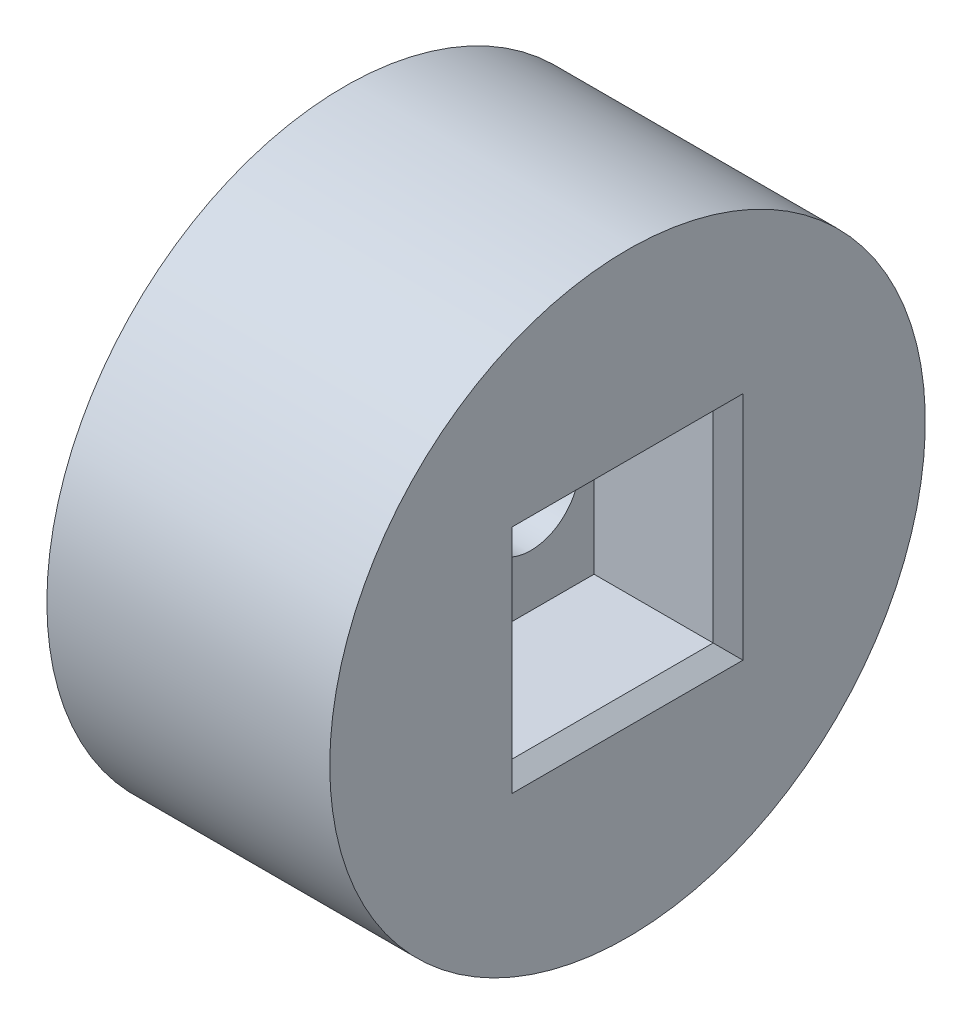
from build123d import *

# Parameters (mm, degrees)
SKETCH1_W                                           = 19
SKETCH1_H                                           = 20
SKETCH2_W                                           = 13.5
SKETCH2_H                                           = 13.5
CUT_EXTRUDE1_DEPTH                                  = 9
CBORE_FOR_M3_HEX_SOCKET_HEAD_CAP_SCREW1_D           = 3.4
CBORE_FOR_M3_HEX_SOCKET_HEAD_CAP_SCREW1_CBORE_D     = 6.5
CBORE_FOR_M3_HEX_SOCKET_HEAD_CAP_SCREW1_CBORE_DEPTH = 3.5
CUT_EXTRUDE2_DEPTH                                  = 31
SKETCH6_R                                           = 5.2
CUT_EXTRUDE3_DEPTH                                  = 3
CHAMFER1_SIZE                                       = 0.5
CHAMFER2_SIZE                                       = 1


with BuildPart() as part:
    # Sketch1 → Revolve1 (revolve)
    with BuildSketch(Plane(origin=(0, 0, 0), x_dir=(1, 0, 0), z_dir=(0, 1, 0))):
        with Locations((9.5, -10)):
            Rectangle(SKETCH1_W, SKETCH1_H)
    revolve(axis=Axis((0, 0, 0), (1, 0, 0)))

    # Sketch2 → Cut-Extrude1 (cut)
    with BuildSketch(Plane(origin=(19, 0, 0), x_dir=(0, 0, -1), z_dir=(1, 0, 0))):
        Rectangle(SKETCH2_W, SKETCH2_H)
    extrude(amount=-CUT_EXTRUDE1_DEPTH, mode=Mode.SUBTRACT)

    # CBORE for M3 Hex Socket Head Cap Screw1 (through all)
    with Locations(Plane(origin=(10, 0, 0), x_dir=(0, 0, -1), z_dir=(1, 0, 0))):
        with Locations((2.5, 0)):
            CounterBoreHole(CBORE_FOR_M3_HEX_SOCKET_HEAD_CAP_SCREW1_D / 2, CBORE_FOR_M3_HEX_SOCKET_HEAD_CAP_SCREW1_CBORE_D / 2, CBORE_FOR_M3_HEX_SOCKET_HEAD_CAP_SCREW1_CBORE_DEPTH)

    # Sketch5 → Cut-Extrude2 (cut, through all)
    with BuildSketch(Plane(origin=(10, 0, 0), x_dir=(0, 0, -1), z_dir=(1, 0, 0))):
        with BuildLine():
            Line((-2, -1), (-4, -1))
            ThreePointArc((-4, -1), (-5, 0), (-4, 1))
            Line((-4, 1), (-2, 1))
            ThreePointArc((-2, 1), (-1, 0), (-2, -1))
        make_face()
    extrude(amount=-CUT_EXTRUDE2_DEPTH, mode=Mode.SUBTRACT)

    # Sketch6 → Cut-Extrude3 (cut)
    with BuildSketch(Plane.ZY):
        Circle(SKETCH6_R)
    extrude(amount=-CUT_EXTRUDE3_DEPTH, mode=Mode.SUBTRACT)

    # Chamfer1
    chamfer1_edges = [part.edges().sort_by_distance(p)[0] for p in [
        (0, 0, -5.2),
    ]]
    chamfer(chamfer1_edges, length=CHAMFER1_SIZE)

    # Chamfer2
    chamfer2_edges = [part.edges().sort_by_distance(p)[0] for p in [
        (19, 0, 6.75),
        (19, -6.75, 0),
        (19, 0, -6.75),
        (19, 6.75, 0),
    ]]
    chamfer(chamfer2_edges, length=CHAMFER2_SIZE)


solid = part.part
